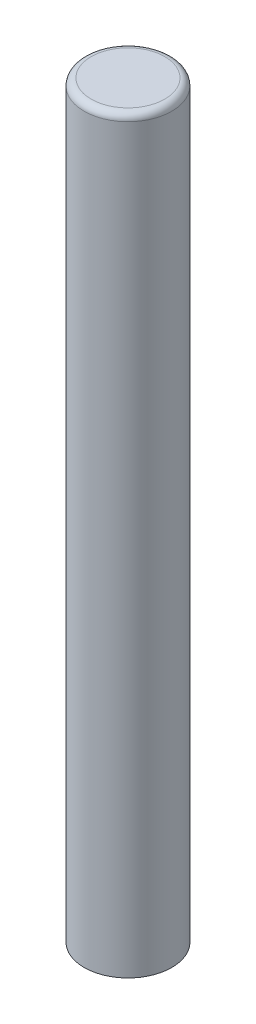
SolidWorks part; units mm, degrees
material "20#"
ref_plane "Front Plane" through (0, 0, 0) normal (0, 0, 1) x (1, 0, 0)
ref_plane "Top Plane" through (0, 0, 0) normal (0, 1, 0) x (1, 0, 0)
ref_plane "Right Plane" through (0, 0, 0) normal (1, 0, 0) x (0, 0, -1)
sketch "Sketch1" plane through (0, 0, 0) normal (0, 1, 0) x (1, 0, 0)
  circle A0 centre (0, 0) radius 12.5
  dimension "D1" = 25
extrude "Boss-Extrude1" add sketch "Sketch1" along normal blind 213.5
fillet "Fillet1" radius 2 1 edges at (0, 213.5, 12.5)
